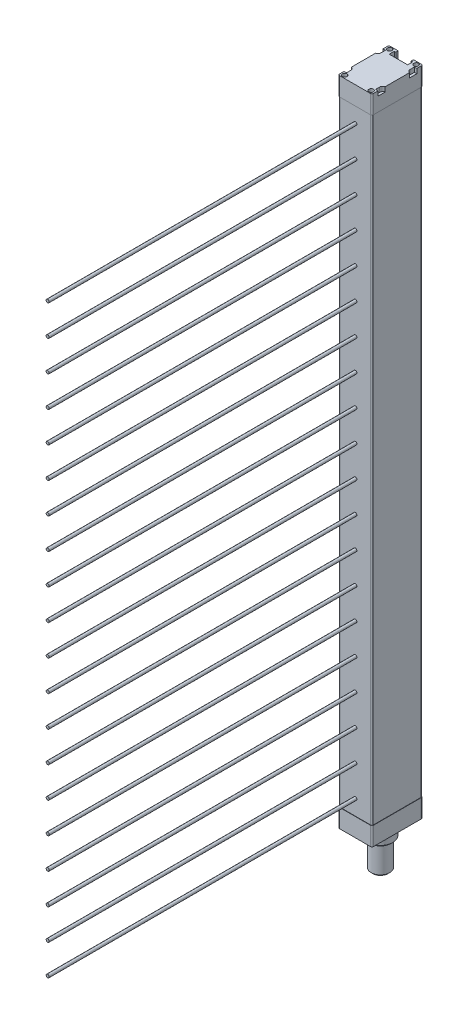
from build123d import *

# Parameters (mm, degrees)
SKETCH_1_R             = 1.5
EXTRUDE_1_DEPTH        = 12
CUT_EXTRUDE_2_DEPTH    = 3
EXTRUDE_3_DEPTH        = 400
SKETCH_5_R             = 1
EXTRUDE_4_DEPTH        = 200
PATTERN_LINEAR_1_COUNT = 20
PATTERN_LINEAR_1_PITCH = 20


with BuildPart() as part:
    # 草圖1 → 伸長1 (new body)
    with BuildSketch(Plane(origin=(0, 0, 0), x_dir=(1, 0, 0), z_dir=(0, 1, 0))):
        with BuildLine():
            Line((-10, 16.5), (-5, 16.5))
            Line((-5, 16.5), (-5, 15))
            Line((-5, 15), (-6, 15))
            Line((-6, 15), (-6, 11.7))
            Line((-6, 11.7), (6, 11.7))
            Line((6, 11.7), (6, 15))
            Line((6, 15), (5, 15))
            Line((5, 15), (5, 16.5))
            Line((5, 16.5), (10, 16.5))
            ThreePointArc((10, 16.5), (10.707106781, 16.207106781), (11, 15.5))
            Line((11, 15.5), (11, -15.5))
            ThreePointArc((11, -15.5), (10.707106781, -16.207106781), (10, -16.5))
            Line((10, -16.5), (-10, -16.5))
            ThreePointArc((-10, -16.5), (-10.707106781, -16.207106781), (-11, -15.5))
            Line((-11, -15.5), (-11, 15.5))
            ThreePointArc((-11, 15.5), (-10.707106781, 16.207106781), (-10, 16.5))
        make_face()
        with Locations(Location((-8.6, 14.6, 0), (0, 0, 270))):
            Circle(SKETCH_1_R, mode=Mode.SUBTRACT)
        with Locations(Location((8.6, 14.6, 0), (0, 0, 90))):
            Circle(SKETCH_1_R, mode=Mode.SUBTRACT)
        with Locations(Location((8.6, -14.6, 0), (0, 0, 270))):
            Circle(SKETCH_1_R, mode=Mode.SUBTRACT)
        with Locations(Location((-8.6, -14.6, 0), (0, 0, 90))):
            Circle(SKETCH_1_R, mode=Mode.SUBTRACT)
    extrude_1 = extrude(amount=EXTRUDE_1_DEPTH)

    # 草圖2 → 伸長2 (cut)
    with BuildSketch(Plane(origin=(0, 12, 0), x_dir=(1, 0, 0), z_dir=(0, 1, 0))):
        with BuildLine():
            Line((-14.2, 12.65), (-9.4, 12.65))
            Line((-9.4, 12.65), (-9.4, 9.85))
            ThreePointArc((-9.4, 9.85), (-9.985786438, 8.435786438), (-11.4, 7.85))
            Line((-11.4, 7.85), (-14.2, 7.85))
            Line((-14.2, 7.85), (-14.2, 12.65))
        make_face()
        with BuildLine():
            Line((9.4, 12.65), (9.4, 9.85))
            ThreePointArc((9.4, 9.85), (9.985786438, 8.435786438), (11.4, 7.85))
            Line((11.4, 7.85), (14.2, 7.85))
            Line((14.2, 7.85), (14.2, 12.65))
            Line((14.2, 12.65), (9.4, 12.65))
        make_face()
        with BuildLine():
            Line((14.2, -12.65), (9.4, -12.65))
            Line((9.4, -12.65), (9.4, -9.85))
            ThreePointArc((9.4, -9.85), (9.985786438, -8.435786438), (11.4, -7.85))
            Line((11.4, -7.85), (14.2, -7.85))
            Line((14.2, -7.85), (14.2, -12.65))
        make_face()
        with BuildLine():
            Line((-9.4, -12.65), (-9.4, -9.85))
            ThreePointArc((-9.4, -9.85), (-9.985786438, -8.435786438), (-11.4, -7.85))
            Line((-11.4, -7.85), (-14.2, -7.85))
            Line((-14.2, -7.85), (-14.2, -12.65))
            Line((-14.2, -12.65), (-9.4, -12.65))
        make_face()
    extrude(amount=-CUT_EXTRUDE_2_DEPTH, mode=Mode.SUBTRACT)

    # 草圖3 → 伸長3 (add)
    with BuildSketch(Plane.XZ):
        with BuildLine():
            Line((-5.2, -16.3), (-5.2, -15.2))
            Line((-5.2, -15.2), (-6.2, -15.2))
            Line((-6.2, -15.2), (-6.2, -11.5))
            Line((-6.2, -11.5), (6.2, -11.5))
            Line((6.2, -11.5), (6.2, -15.2))
            Line((6.2, -15.2), (5.2, -15.2))
            Line((5.2, -15.2), (5.2, -16.3))
            Line((5.2, -16.3), (10, -16.3))
            ThreePointArc((10, -16.3), (10.565685425, -16.065685425), (10.8, -15.5))
            Line((10.8, -15.5), (10.8, 15.5))
            ThreePointArc((10.8, 15.5), (10.565685425, 16.065685425), (10, 16.3))
            Line((10, 16.3), (-10, 16.3))
            ThreePointArc((-10, 16.3), (-10.565685425, 16.065685425), (-10.8, 15.5))
            Line((-10.8, 15.5), (-10.8, -15.5))
            ThreePointArc((-10.8, -15.5), (-10.565685425, -16.065685425), (-10, -16.3))
            Line((-10, -16.3), (-5.2, -16.3))
        make_face()
    extrude(amount=EXTRUDE_3_DEPTH)

    # 鏡射1: 伸長1 across plane
    add(extrude_1.mirror(Plane.ZX.offset(-200)))

    # 草圖4 → 旋轉1 (revolve)
    with BuildSketch(Plane(origin=(0, 0, 0), x_dir=(0, 0, -1), z_dir=(1, 0, 0))):
        Polygon((8, -412), (8, -419), (7, -419), (7, -420), (6, -420), (6, -437), (5, -438), (0, -438), (0, -412), align=None)
    revolve(axis=Axis((0, -412, 0), (0, 1, 0)))

    # 草圖5 → 伸長4 (add)
    with BuildSketch(Plane.XY.offset(16.3)):
        with Locations(Location((0, -10, 0), (0, 0, 180))):
            Circle(SKETCH_5_R)
    extrude_4 = extrude(amount=EXTRUDE_4_DEPTH)

    # 阵列(线性)1: 伸長4 ×20
    with Locations(*[(0, -i * PATTERN_LINEAR_1_PITCH, 0) for i in range(1, PATTERN_LINEAR_1_COUNT)]):
        add(extrude_4)


solid = part.part
